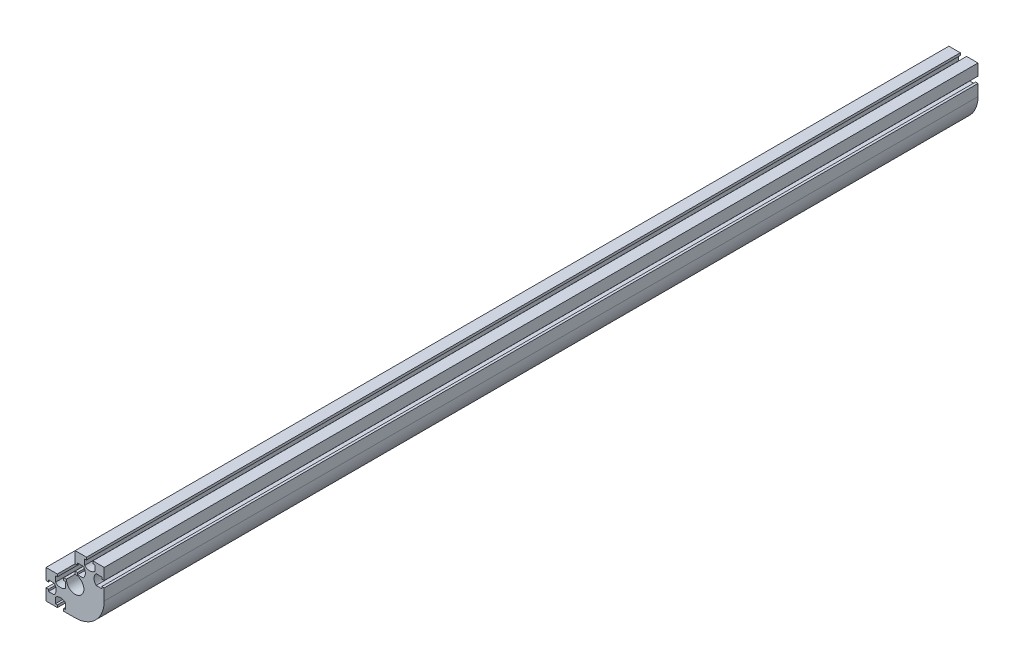
from build123d import *

# Parameters (mm, degrees)
EXTRUDE_1_DEPTH = 900


with BuildPart() as part:
    # 草图1 → 凸台-拉伸1 (new body)
    with BuildSketch(Plane.XY):
        with BuildLine():
            Line((0, 9), (0, 11.75))
            Line((0, 11.75), (2.5, 11.75))
            Line((2.5, 11.75), (2.5, 9.75))
            Line((2.5, 9.75), (8.36, 9.75))
            ThreePointArc((8.36, 9.75), (10.502806142, 15), (8.36, 20.25))
            Line((8.36, 20.25), (2.5, 20.25))
            Line((2.5, 20.25), (2.5, 18.25))
            Line((2.5, 18.25), (0, 18.25))
            Line((0, 18.25), (0, 30))
            Line((0, 30), (11.75, 30))
            Line((11.75, 30), (11.75, 27.5))
            Line((11.75, 27.5), (9.75, 27.5))
            Line((9.75, 27.5), (9.75, 21.64))
            ThreePointArc((9.75, 21.64), (15, 19.497193858), (20.25, 21.64))
            Line((20.25, 21.64), (20.25, 27.5))
            Line((20.25, 27.5), (18.25, 27.5))
            Line((18.25, 27.5), (18.25, 30))
            Line((18.25, 30), (30, 30))
            Line((30, 30), (30, 18.25))
            Line((30, 18.25), (27.5, 18.25))
            Line((27.5, 18.25), (27.5, 20.25))
            Line((27.5, 20.25), (21.64, 20.25))
            ThreePointArc((21.64, 20.25), (19.497193858, 15), (21.64, 9.75))
            Line((21.64, 9.75), (27.5, 9.75))
            Line((27.5, 9.75), (27.5, 11.75))
            Line((27.5, 11.75), (30, 11.75))
            Line((30, 11.75), (30, 0))
            ThreePointArc((30, 0), (21.213203436, -21.213203436), (0, -30))
            Line((0, -30), (-11.75, -30))
            Line((-11.75, -30), (-11.75, -27.5))
            Line((-11.75, -27.5), (-9.75, -27.5))
            Line((-9.75, -27.5), (-9.75, -21.64))
            ThreePointArc((-9.75, -21.64), (-15, -19.497193858), (-20.25, -21.64))
            Line((-20.25, -21.64), (-20.25, -27.5))
            Line((-20.25, -27.5), (-18.25, -27.5))
            Line((-18.25, -27.5), (-18.25, -30))
            Line((-18.25, -30), (-30, -30))
            Line((-30, -30), (-30, -18.25))
            Line((-30, -18.25), (-27.5, -18.25))
            Line((-27.5, -18.25), (-27.5, -20.25))
            Line((-27.5, -20.25), (-21.64, -20.25))
            ThreePointArc((-21.64, -20.25), (-19.497193858, -15), (-21.64, -9.75))
            Line((-21.64, -9.75), (-27.5, -9.75))
            Line((-27.5, -9.75), (-27.5, -11.75))
            Line((-27.5, -11.75), (-30, -11.75))
            Line((-30, -11.75), (-30, 0))
            Line((-30, 0), (-18.25, 0))
            Line((-18.25, 0), (-18.25, -2.5))
            Line((-18.25, -2.5), (-20.25, -2.5))
            Line((-20.25, -2.5), (-20.25, -8.36))
            ThreePointArc((-20.25, -8.36), (-15, -10.502806142), (-9.75, -8.36))
            Line((-9.75, -8.36), (-9.75, -2.5))
            Line((-9.75, -2.5), (-11.75, -2.5))
            Line((-11.75, -2.5), (-11.75, 0))
            Line((-11.75, 0), (-9, 0))
            ThreePointArc((-9, 0), (6.363961031, -6.363961031), (0, 9))
        make_face()
    extrude(amount=EXTRUDE_1_DEPTH)


solid = part.part
